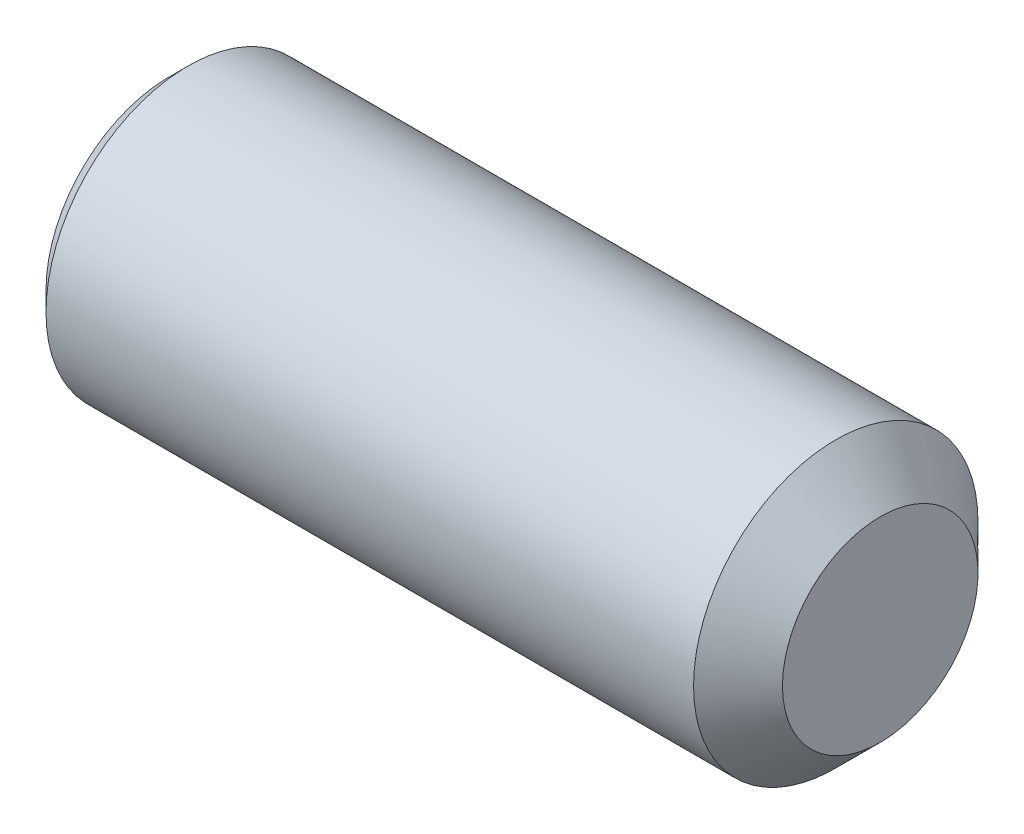
from build123d import *

# Parameters (mm, degrees)
CUT_EXTRUDE_1_DEPTH = 5


with BuildPart() as part:
    # 草图1 → Revolve 587 (revolve)
    with BuildSketch(Plane.XY, mode=Mode.PRIVATE) as revolve_587_sk:
        Polygon((0, 0), (20, 0), (20, 2.75), (18.75, 4), (0.536, 4), (0, 3.464), align=None)
    revolve(revolve_587_sk.sketch.rotate(Axis((-0.277777778, 0, 0), (1, 0, 0)), 90), axis=Axis((-0.277777778, 0, 0), (1, 0, 0)))

    # 草图2 → 切除-拉伸1 (cut)
    with BuildSketch(Plane.ZY):
        Polygon((-1.154700538, -2), (1.154700538, -2), (2.309401077, 0), (1.154700538, 2), (-1.154700538, 2), (-2.309401077, 0), align=None)
    extrude(amount=-CUT_EXTRUDE_1_DEPTH, mode=Mode.SUBTRACT)

    # 草图4 → 切除-旋转2 (revolve, cut)
    with BuildSketch(Plane.XY, mode=Mode.PRIVATE) as cut_revolve_2_sk:
        Polygon((5, 2), (6.154700538, 0), (5, 0), align=None)
    revolve(cut_revolve_2_sk.sketch.rotate(Axis((-0.277777778, 0, 0), (1, 0, 0)), 90), axis=Axis((-0.277777778, 0, 0), (1, 0, 0)), mode=Mode.SUBTRACT)


solid = part.part
